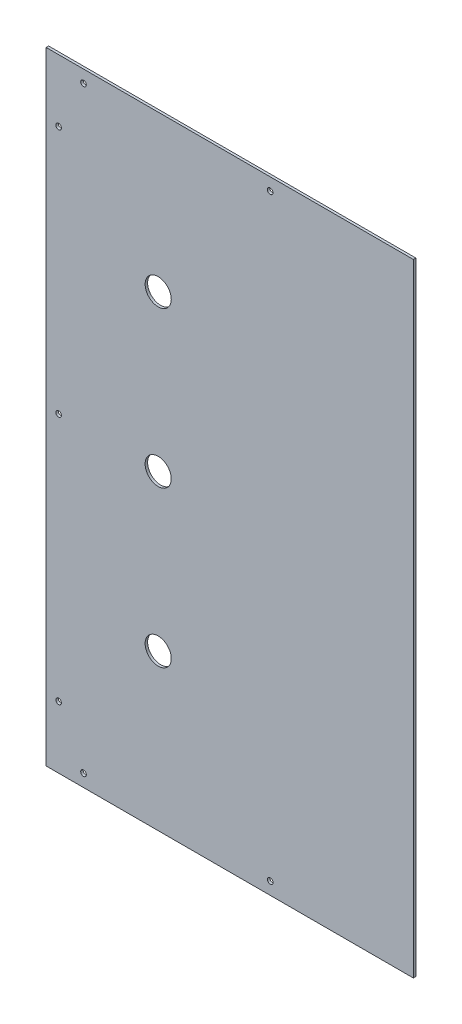
SolidWorks part; units mm, degrees
material "Q235A"
ref_plane "前视基准面" through (0, 0, 0) normal (0, 0, 1) x (1, 0, 0)
ref_plane "上视基准面" through (0, 0, 0) normal (0, 1, 0) x (1, 0, 0)
ref_plane "右视基准面" through (0, 0, 0) normal (1, 0, 0) x (0, 0, -1)
sketch "草图1" plane through (0, 0, 0) normal (0, 0, 1) x (1, 0, 0)
  line L1 (-147.5, 250) -> (147.5, 250)
  line L2 (-147.5, 250) -> (-147.5, -250)
  line L3 (-147.5, -250) -> (147.5, -250)
  line L4 (147.5, 250) -> (147.5, -250)
  line L5 (0, -250) -> (0, 250) construction
  line L6 (-147.5, 0) -> (147.5, 0) construction
  point P0 (0, 0)
  dimension "D1" = 295
  dimension "D2" = 500
extrude "凸台-拉伸1" add sketch "草图1" along normal blind 2
hole_wizard "Ø4.5 (4.5) 直径孔1" positions "草图2" profile "草图3" hole size "Ø4.5" standard "GB"
sketch "草图2" plane through (0, 0, 2) normal (0, 0, 1) x (1, 0, 0)
  line L1 (-137.5, -240) -> (62.5, -240) construction
  line L2 (-137.5, -240) -> (-137.5, 240) construction
  line L3 (-137.5, 240) -> (62.5, 240) construction
  line L4 (62.5, -240) -> (62.5, 240) construction
  line L5 (-37.5, 240) -> (-37.5, -240) construction
  line L6 (-137.5, 0) -> (62.5, 0) construction
  line L7 (-147.5, 250) -> (-147.5, -250) construction
  point P330 (-137.5, 0)
  point P336 (-137.5, 200)
  point P341 (-137.5, -200)
  point P342 (-117.5, 240)
  point P344 (32.5, 240)
  point P347 (32.5, -240)
  point P348 (-117.5, -240)
  dimension "D1" = 200
  dimension "D2" = 480
  dimension "D3" = 150
  dimension "D4" = 200
  dimension "D5" = 20
  dimension "D6" = 10
sketch "草图3" plane through (-117.5, -240, 2) normal (1, 0, 0) x (0, -1, 0)
  line L0 (0, 0) -> (0, 9.3519)
  line L1 (0, 9.3519) -> (2.25, 8)
  line L2 (2.25, 8) -> (2.25, 0)
  line L5 (2.25, 0) -> (0, 0)
  line L10 (0, 9.3519) -> (-2.25, 8) construction
  line L11 (0, -6.35) -> (0, 107.95) construction
  dimension "孔直径" = 4.5
  dimension "孔深度" = 8
  dimension "导头角度" = 118
sketch "草图4" plane through (0, 0, 2) normal (0, 0, 1) x (1, 0, 0)
  line L0 (-147.5, 0) -> (147.5, 0) construction
  line L1 (-147.5, 250) -> (-147.5, -250) construction
  line L2 (147.5, -250) -> (147.5, 250) construction
  line L3 (-78.5829, 250) -> (-78.5829, 199.6769) construction
  line L4 (147.5, 250) -> (-147.5, 250) construction
  line L5 (-57.5, -250) -> (-57.5, 250) construction
  circle A0 centre (-57.5, 125) radius 10.5
  circle A1 centre (-57.5, -125) radius 10.5
  circle A3 centre (-57.5, 0) radius 10.5
  dimension "D2" = 21
  dimension "D1" = 90
  dimension "D3" = 250
extrude "切除-拉伸1" cut sketch "草图4" against normal blind 10
